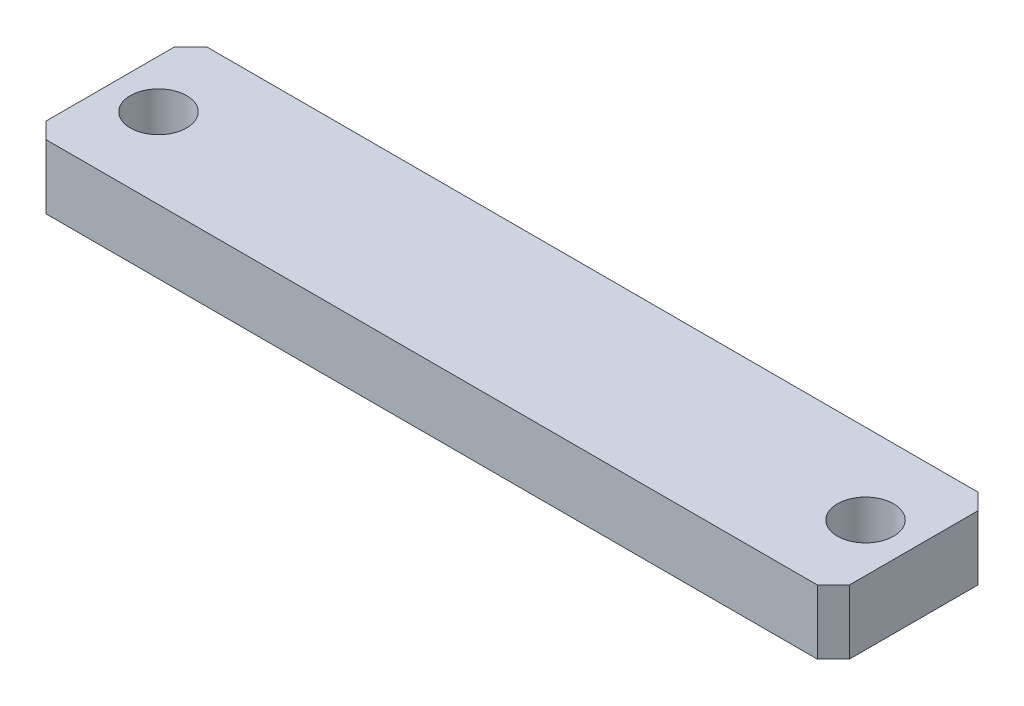
SolidWorks part; units mm, degrees
ref_plane "Front Plane" through (0, 0, 0) normal (0, 0, 1) x (1, 0, 0)
ref_plane "Top Plane" through (0, 0, 0) normal (0, 1, 0) x (1, 0, 0)
ref_plane "Right Plane" through (0, 0, 0) normal (1, 0, 0) x (0, 0, -1)
sketch "Sketch1" plane through (0, 0, 0) normal (0, 1, 0) x (1, 0, 0)
  line L1 (-25, 5) -> (25, 5)
  line L2 (-25, 5) -> (-25, -5)
  line L3 (-25, -5) -> (25, -5)
  line L4 (25, 5) -> (25, -5)
  line L5 (-25, 5) -> (25, -5) construction
  line L6 (-25, -5) -> (25, 5) construction
  point P0 (0, 0)
  dimension "D1" = 50
  dimension "D2" = 10
extrude "Boss-Extrude1" add sketch "Sketch1" along normal mid plane 4
hole_wizard "Ø3.5 (3.5) Diameter Hole1" positions "Sketch3" profile "Sketch2" hole size "Ø3.5" standard "Gb" end condition through all
sketch "Sketch3" plane through (0, 2, 0) normal (0, 1, 0) x (1, 0, 0)
  line L0 (0, 0) -> (0, 12.3226) construction
  line L2 (25, -5) -> (25, 5) construction
  point P0 (-22, 0)
  point P2 (22, 0)
  dimension "D1" = 3
sketch "Sketch2" plane through (-22, 2, 0) normal (1, 0, 0) x (0, 0, 1)
  line L0 (0, 0) -> (0, 4)
  line L1 (0, 4) -> (1.75, 4)
  line L2 (1.75, 4) -> (1.75, 0)
  line L5 (1.75, 0) -> (0, 0)
  line L11 (0, -6.35) -> (0, 107.95) construction
  dimension "通孔孔直径" = 3.5
  dimension "通孔孔深度" = 4
chamfer "Chamfer1" distance 1 angle 45 4 edges at (25, 0, -5) (25, 0, 5) (-25, 0, -5) (-25, 0, 5)
sketch "Sketch4" plane through (0, -2, 0) normal (0, -1, 0) x (1, 0, 0)
  line L1 (-17, 3.5) -> (17, 3.5)
  line L2 (-19, 1.5) -> (-19, -1.5)
  line L3 (-17, -3.5) -> (17, -3.5)
  line L4 (19, 1.5) -> (19, -1.5)
  line L5 (-19, 3.5) -> (19, -3.5) construction
  line L6 (-19, -3.5) -> (19, 3.5) construction
  arc A0 (17, 3.5) -> (19, 1.5) centre (17, 1.5) cw
  arc A1 (19, -1.5) -> (17, -3.5) centre (17, -1.5) cw
  arc A2 (-17, -3.5) -> (-19, -1.5) centre (-17, -1.5) cw
  arc A3 (-17, 3.5) -> (-19, 1.5) centre (-17, 1.5) ccw
  point P0 (0, 0)
  dimension "D3" = 2
  dimension "D1" = 38
  dimension "D2" = 7
extrude "Cut-Extrude1" cut sketch "Sketch4" against normal blind 2
